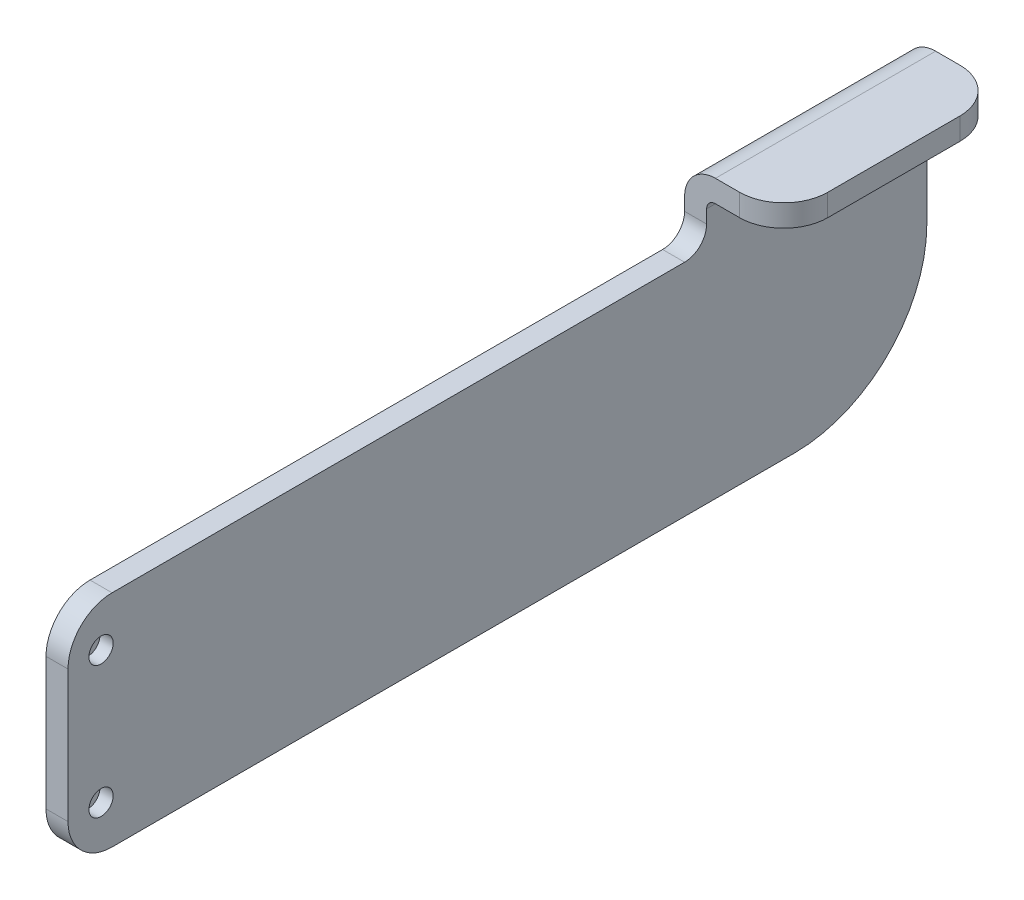
from build123d import *

# Parameters (mm, degrees)
EXTRUDE_THIN1_DEPTH = 100
SKETCH2_W           = 10
SKETCH2_H           = 100
BOSS_EXTRUDE1_DEPTH = 290
FILLET1_R           = 10
FILLET3_R           = 20
FILLET4_R           = 60
SKETCH3_R           = 6
CUT_EXTRUDE1_DEPTH  = 6
LPATTERN1_COUNT     = 2
LPATTERN1_PITCH     = 70
SKETCH4_R           = 5.5
CUT_EXTRUDE2_DEPTH  = 6
LPATTERN2_COUNT     = 2
LPATTERN2_PITCH     = 60


with BuildPart() as part:
    # Sketch1 → Extrude-Thin1 (new body)
    with BuildSketch(Plane.XY):
        with BuildLine():
            Line((0, -130), (0, -14))
            ThreePointArc((0, -14), (4.100505063, -4.100505063), (14, 0))
            Line((14, 0), (45, 0))
            Line((45, 0), (45, -10))
            Line((45, -10), (14, -10))
            ThreePointArc((14, -10), (11.171572875, -11.171572875), (10, -14))
            Line((10, -14), (10, -130))
            Line((10, -130), (0, -130))
        make_face()
    extrude(amount=EXTRUDE_THIN1_DEPTH)

    # Sketch2 → Boss-Extrude1 (add)
    with BuildSketch(Plane.XY.offset(100)):
        with Locations((5, -80)):
            Rectangle(SKETCH2_W, SKETCH2_H)
    extrude(amount=BOSS_EXTRUDE1_DEPTH)

    # Fillet1
    fillet1_edges = [part.edges().sort_by_distance(p)[0] for p in [
        (5, -30, 100),
    ]]
    fillet(fillet1_edges, radius=FILLET1_R)

    # Fillet3
    fillet3_edges = [part.edges().sort_by_distance(p)[0] for p in [
        (5, -30, 390),
        (5, -130, 390),
        (45, -5, 0),
        (45, -5, 100),
    ]]
    fillet(fillet3_edges, radius=FILLET3_R)

    # Fillet4
    fillet4_edges = [part.edges().sort_by_distance(p)[0] for p in [
        (5, -130, 0),
    ]]
    fillet(fillet4_edges, radius=FILLET4_R)

    # Sketch3 → Cut-Extrude1 (cut)
    with BuildSketch(Plane.XZ.offset(10)):
        with Locations(Location((30, 15, 0), (0, 0, 270))):
            Circle(SKETCH3_R)
    cut_extrude1 = extrude(amount=-CUT_EXTRUDE1_DEPTH, mode=Mode.SUBTRACT)

    # LPattern1: Cut-Extrude1 ×2
    with Locations(*[(0, 0, i * LPATTERN1_PITCH) for i in range(1, LPATTERN1_COUNT)]):
        add(cut_extrude1, mode=Mode.SUBTRACT)

    # Sketch4 → Cut-Extrude2 (cut)
    with BuildSketch(Plane(origin=(10, 0, 0), x_dir=(0, 0, -1), z_dir=(1, 0, 0))):
        with Locations(Location((-375, -50, 0), (0, 0, 90))):
            Circle(SKETCH4_R)
    cut_extrude2 = extrude(amount=-CUT_EXTRUDE2_DEPTH, mode=Mode.SUBTRACT)

    # LPattern2: Cut-Extrude2 ×2
    with Locations(*[(0, -i * LPATTERN2_PITCH, 0) for i in range(1, LPATTERN2_COUNT)]):
        add(cut_extrude2, mode=Mode.SUBTRACT)


solid = part.part
